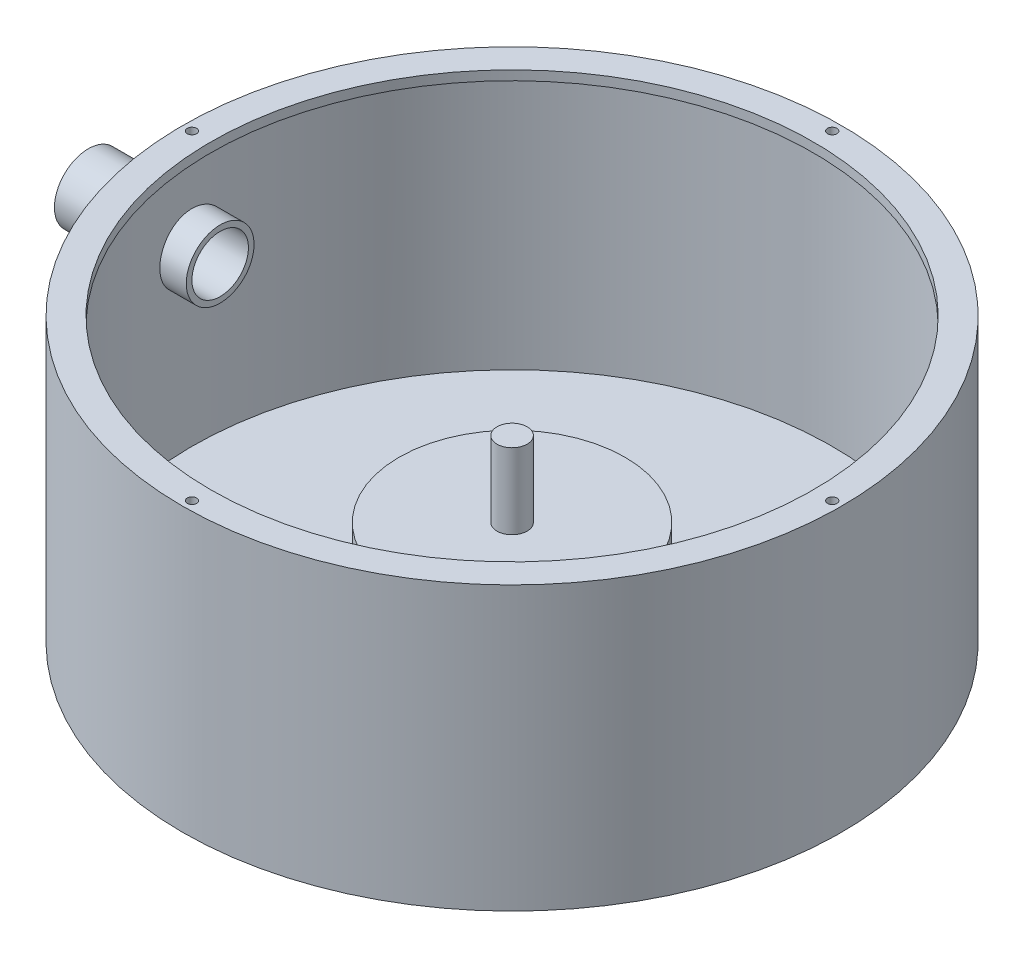
from build123d import *

# Parameters (mm, degrees)
SKETCH1_R                = 175
BOSS_EXTRUDE2_DEPTH      = 150
SHELL2_T                 = -5
SKETCH2_R                = 60
BOSS_EXTRUDE3_DEPTH      = 50
SKETCH_3_3_R             = 15
CUT_EXTRUDE1_DEPTH       = 50
BOSS_EXTRUDE5_DEPTH      = 50
BOSS_EXTRUDE5_DEPTH_BACK = 20
SKETCH_3_3_2_R           = 18
SKETCH_3_3_2_R_2         = 15
SKETCH5_R                = 8
BOSS_EXTRUDE6_DEPTH      = 40
BOSS_EXTRUDE7_START      = -5
SKETCH6_R                = 170
SKETCH6_R_2              = 160
BOSS_EXTRUDE7_DEPTH      = 5
SKETCH7_R                = 2.5
CUT_EXTRUDE2_DEPTH       = 10


with BuildPart() as part:
    # Sketch1 → Boss-Extrude2 (new body)
    with BuildSketch(Plane(origin=(0, 0, 0), x_dir=(1, 0, 0), z_dir=(0, 1, 0))):
        with Locations(Location((0, 0, 0), (0, 0, 270))):
            Circle(SKETCH1_R)
    extrude(amount=BOSS_EXTRUDE2_DEPTH)

    # Shell2
    shell2_openings = [part.faces().sort_by_distance(p)[0] for p in [
        (0, 150, 0),
    ]]
    offset(amount=SHELL2_T, openings=shell2_openings, kind=Kind.INTERSECTION)

    # Sketch2 → Boss-Extrude3 (add)
    with BuildSketch(Plane(origin=(0, 5, 0), x_dir=(1, 0, 0), z_dir=(0, 1, 0))):
        with Locations(Location((0, 0, 0), (0, 0, 270))):
            Circle(SKETCH2_R)
    extrude(amount=BOSS_EXTRUDE3_DEPTH)

    # Sketch 3_3 → Cut-Extrude1 (cut)
    with BuildSketch(Plane.ZY.offset(175)):
        with Locations((0, 96.363123984)):
            Circle(SKETCH_3_3_R)
    extrude(amount=-CUT_EXTRUDE1_DEPTH, mode=Mode.SUBTRACT)

    # Sketch 3_3 2 → Boss-Extrude5 (add, two sides: drawn at the far end of the back side and taken through both)
    with BuildSketch(Plane.ZY.offset(175).offset(-BOSS_EXTRUDE5_DEPTH_BACK)):
        with Locations((0, 96.363123984)):
            Circle(SKETCH_3_3_2_R)
        with Locations((0, 96.363123984)):
            Circle(SKETCH_3_3_2_R_2, mode=Mode.SUBTRACT)
    extrude(amount=BOSS_EXTRUDE5_DEPTH + BOSS_EXTRUDE5_DEPTH_BACK)

    # Sketch5 → Boss-Extrude6 (add)
    with BuildSketch(Plane(origin=(0, 55, 0), x_dir=(1, 0, 0), z_dir=(0, 1, 0))):
        with Locations(Location((0, 0, 0), (0, 0, 270))):
            Circle(SKETCH5_R)
    extrude(amount=BOSS_EXTRUDE6_DEPTH)

    # Sketch6 → Boss-Extrude7 (add)
    with BuildSketch(Plane(origin=(0, 150, 0), x_dir=(1, 0, 0), z_dir=(0, 1, 0)).offset(BOSS_EXTRUDE7_START)):
        with Locations(Location((0, 0, 0), (0, 0, 270))):
            Circle(SKETCH6_R)
        with Locations(Location((0, 0, 0), (0, 0, 270))):
            Circle(SKETCH6_R_2, mode=Mode.SUBTRACT)
    extrude(amount=BOSS_EXTRUDE7_DEPTH)

    # Sketch7 → Cut-Extrude2 (cut)
    with BuildSketch(Plane(origin=(0, 150, 0), x_dir=(1, 0, 0), z_dir=(0, 1, 0))):
        with Locations(Location((0, -170, 0), (0, 0, 270))):
            Circle(SKETCH7_R)
        with Locations(Location((-170, 0, 0), (0, 0, 270))):
            Circle(SKETCH7_R)
        with Locations(Location((0, 170, 0), (0, 0, 270))):
            Circle(SKETCH7_R)
        with Locations(Location((170, 0, 0), (0, 0, 270))):
            Circle(SKETCH7_R)
    extrude(amount=-CUT_EXTRUDE2_DEPTH, mode=Mode.SUBTRACT)


solid = part.part
